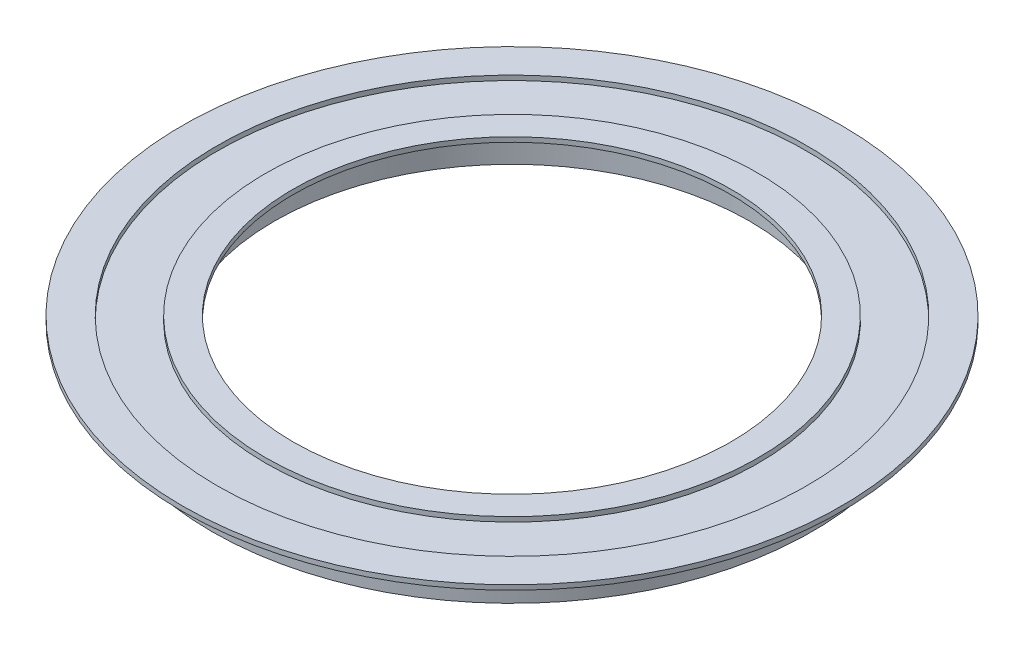
from build123d import *

# Parameters (mm, degrees)
SKETCH1_W = 5.771968746
SKETCH1_H = 1


with BuildPart() as part:
    # Sketch1 → Revolve1 (revolve)
    with BuildSketch(Plane.XY, mode=Mode.PRIVATE) as revolve1_sk:
        Polygon((63.193534924, 160.531936258), (69.363427474, 160.531936258), (69.363427474, 161.531936258), (62.033691631, 161.531936258), (62.033691631, 160.531936258), (50, 160.531936258), (50, 153.778962031), (63.193534924, 153.778962031), align=None)
        with Locations((48.9671445, 161.068033461)):
            Rectangle(SKETCH1_W, SKETCH1_H)
    revolve(revolve1_sk.sketch.rotate(Axis((0, 0, 0), (0, -1, 0)), 90), axis=Axis((0, 0, 0), (0, -1, 0)))


solid = part.part
